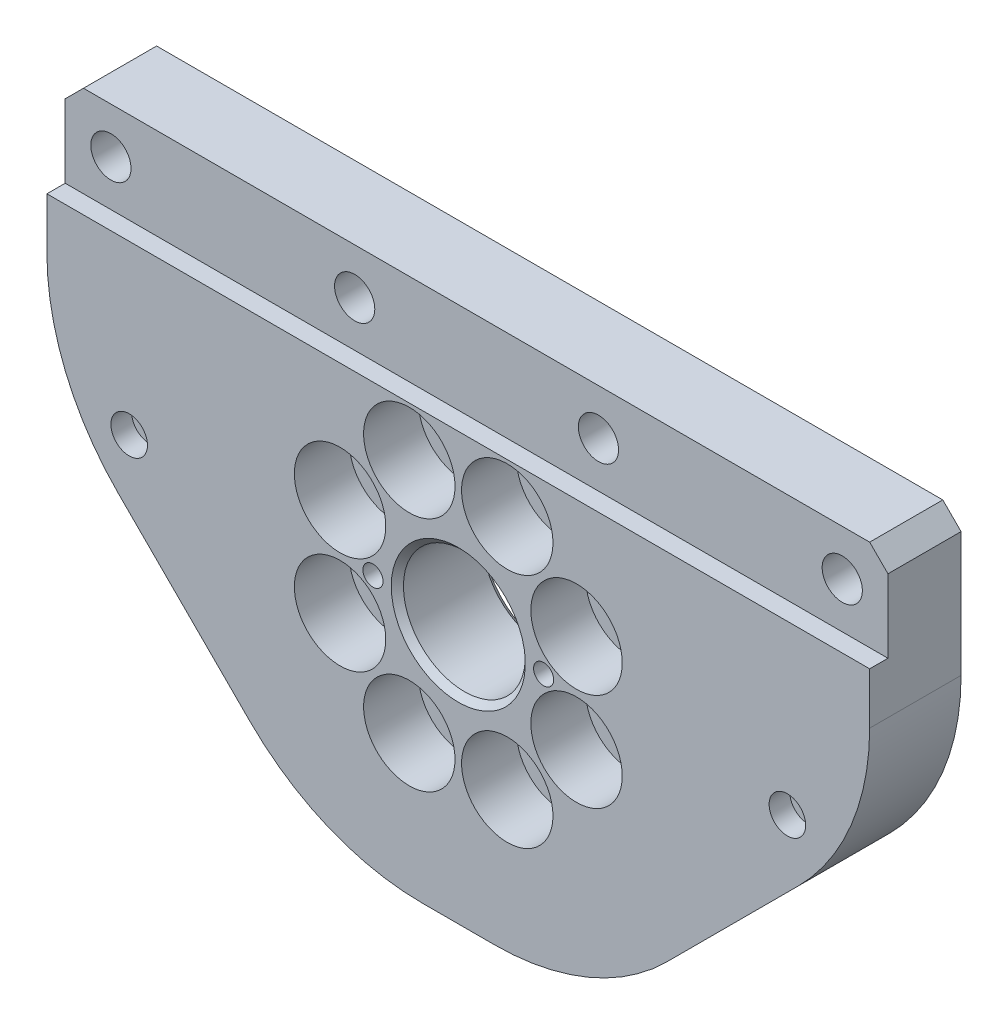
SolidWorks part; units mm, degrees
material "AL6061"
ref_plane "前视基准面" through (0, 0, 0) normal (0, 0, 1) x (1, 0, 0)
ref_plane "上视基准面" through (0, 0, 0) normal (0, 1, 0) x (1, 0, 0)
ref_plane "右视基准面" through (0, 0, 0) normal (1, 0, 0) x (0, 0, -1)
sketch "草图1" plane through (0, 0, 0) normal (0, 0, 1) x (1, 0, 0)
  line L0 (-77.8941, 0) -> (76.4, 0) construction
  line L1 (0, 37.9961) -> (0, -44.0164) construction
  line L2 (-55.7843, -9.2157) -> (-34.2157, -30.7843)
  line L3 (-67.5, 42.5) -> (67.5, 42.5)
  line L4 (-67.5, 42.5) -> (-67.5, 19.0685)
  line L5 (-5.9315, -42.5) -> (5.9315, -42.5)
  line L6 (67.5, 42.5) -> (67.5, 19.0685)
  line L7 (55.7843, -9.2157) -> (34.2157, -30.7843)
  arc A0 (-55.7843, -9.2157) -> (-67.5, 19.0685) centre (-27.5, 19.0685) cw
  arc A1 (-34.2157, -30.7843) -> (-5.9315, -42.5) centre (-5.9315, -2.5) ccw
  arc A2 (34.2157, -30.7843) -> (5.9315, -42.5) centre (5.9315, -2.5) cw
  arc A3 (55.7843, -9.2157) -> (67.5, 19.0685) centre (27.5, 19.0685) ccw
  circle A4 centre (0, 0) radius 10
  point P13 (-67.5, 2.5)
  point P16 (-22.5, -42.5)
  point P19 (22.5, -42.5)
  point P22 (67.5, 2.5)
  dimension "D5" = 40
  dimension "D6" = 42.5
  dimension "D7" = 20
  dimension "D1" = 135
  dimension "D2" = 85
  dimension "D3" = 45
  dimension "D4" = 45
extrude "凸台-拉伸1" add sketch "草图1" along normal mid plane 15
hole_wizard "打孔尺寸(%根据)内六角圆柱头螺钉的类型2" positions "草图2" profile "草图3" counterbore size "M8" standard "GB" end condition through all
sketch "草图2" plane through (0, 0, 7.5) normal (0, 0, 1) x (1, 0, 0)
  line L0 (0, 44.1868) -> (0, -47.6954) construction
  line L1 (0, 0) -> (-24.5604, 0) construction
  line L2 (0, 0) -> (-11.1113, 26.8251) construction
  circle A0 centre (0, 0) radius 21 construction
  point P0 (-8.0364, 19.4015)
  dimension "D1" = 42
  dimension "D2" = 22.5
sketch "草图3" plane through (-8.0364, 19.4015, 7.5) normal (1, 0, 0) x (0, -1, 0)
  line L0 (0, 0) -> (0, 15)
  line L1 (0, 15) -> (4.5, 15)
  line L3 (4.5, 15) -> (4.5, 9)
  line L4 (4.5, 9) -> (7.5, 9)
  line L5 (7.5, 9) -> (7.5, 0)
  line L7 (7.5, 0) -> (0, 0)
  line L11 (0, -6.35) -> (0, 107.95) construction
  dimension "通孔孔直径" = 9
  dimension "通孔孔深度" = 15
  dimension "柱形沉头孔直径" = 15
  dimension "柱形沉头孔深度" = 9
chamfer "倒角1" distance 1 angle 45 2 edges at (10, 0, -7.5) (10, 0, 7.5)
pattern_circular "阵列(圆周)1" count 8 over 360 about axis through (0, 0, 0) along (0, 0, 1) of "打孔尺寸(%根据)内六角圆柱头螺钉的类型2"
hole_wizard "打孔尺寸(%根据)内六角圆柱头螺钉的类型2" positions "草图4" profile "草图5" counterbore size "M3" standard "GB" end condition through all
sketch "草图4" plane through (0, 0, 7.5) normal (0, 0, 1) x (1, 0, 0)
  line L0 (0, 45.6613) -> (0, -51.3453) construction
  line L1 (0, 0) -> (80.3336, 0) construction
  point P0 (-54, 0)
  point P8 (54, 0)
  dimension "D1" = 108
sketch "草图5" plane through (-54, 0, 7.5) normal (1, 0, 0) x (0, -1, 0)
  line L0 (0, 0) -> (0, 15)
  line L1 (0, 15) -> (1.7, 15)
  line L3 (1.7, 15) -> (1.7, 3.4)
  line L4 (1.7, 3.4) -> (3, 3.4)
  line L5 (3, 3.4) -> (3, 0)
  line L7 (3, 0) -> (0, 0)
  line L11 (0, -6.35) -> (0, 107.95) construction
  dimension "通孔孔直径" = 3.4
  dimension "通孔孔深度" = 15
  dimension "柱形沉头孔直径" = 6
  dimension "柱形沉头孔深度" = 3.4
hole_wizard "Ø8.0 (8) 直径孔1" positions "草图6" profile "草图7" hole size "Ø8.0" standard "GB"
sketch "草图6" plane through (0, 0, -7.5) normal (0, 0, -1) x (-1, 0, 0)
  point P0 (-54, 0)
  point P3 (54, 0)
sketch "草图7" plane through (54, 0, -7.5) normal (1, 0, 0) x (0, 1, 0)
  line L0 (0, 0) -> (0, 10.4034)
  line L1 (0, 10.4034) -> (4, 8)
  line L2 (4, 8) -> (4, 0)
  line L5 (4, 0) -> (0, 0)
  line L10 (0, 10.4034) -> (-4, 8) construction
  line L11 (0, -6.35) -> (0, 107.95) construction
  dimension "孔直径" = 8
  dimension "孔深度" = 8
  dimension "导头角度" = 118
hole_wizard "M4 螺纹孔1" positions "草图8" profile "草图9" tap size "M4" standard "GB" end condition through all
sketch "草图8" plane through (0, 0, -7.5) normal (0, 0, -1) x (-1, 0, 0)
  line L0 (0, 0) -> (-34.4162, 0) construction
  line L1 (0, 22.5985) -> (0, -19.4015) construction
  point P0 (-14, 0)
  point P12 (14, 0)
  dimension "D1" = 28
sketch "草图9" plane through (14, 0, -7.5) normal (1, 0, 0) x (0, 1, 0)
  line L0 (0, 0) -> (0, 15)
  line L1 (0, 15) -> (1.65, 15)
  line L2 (1.65, 15) -> (1.65, 0)
  line L5 (1.65, 0) -> (0, 0)
  line L11 (0, -6.35) -> (0, 107.95) construction
  dimension "通孔螺纹孔钻头直径" = 3.3
  dimension "通孔螺纹孔钻头深度" = 15
cosmetic thread "孔螺蚊线1" parameters "D2"=4
cosmetic thread "孔螺蚊线2" parameters "D2"=4
sketch "草图10" plane through (0, 0, 7.5) normal (0, 0, 1) x (1, 0, 0)
  line L0 (67.5, 19.0685) -> (67.5, 42.5) construction
  line L1 (-67.5, 42.5) -> (67.5, 42.5)
  line L2 (-67.5, 42.5) -> (-67.5, 27.5)
  line L3 (-67.5, 27.5) -> (67.5, 27.5)
  line L4 (67.5, 42.5) -> (67.5, 27.5)
  dimension "D1" = 15
extrude "切除-拉伸1" cut sketch "草图10" against normal blind 3
hole_wizard "打孔尺寸(%根据)内六角圆柱头螺钉的类型3" positions "草图11" profile "草图12" counterbore size "M6" standard "GB" end condition through all
sketch "草图11" plane through (0, 0, -7.5) normal (0, 0, -1) x (-1, 0, 0)
  line L0 (0, 44.4035) -> (0, -4.632) construction
  line L1 (-67.5, 42.5) -> (67.5, 42.5) construction
  point P0 (-20, 35)
  point P2 (-60, 35)
  point P9 (60, 35)
  point P10 (20, 35)
  dimension "D1" = 40
  dimension "D2" = 120
  dimension "D3" = 7.5
sketch "草图12" plane through (20, 35, -7.5) normal (1, 0, 0) x (0, 1, 0)
  line L0 (0, 0) -> (0, 15)
  line L1 (0, 15) -> (3.3, 15)
  line L3 (3.3, 15) -> (3.3, 6.8)
  line L4 (3.3, 6.8) -> (5.5, 6.8)
  line L5 (5.5, 6.8) -> (5.5, 0)
  line L7 (5.5, 0) -> (0, 0)
  line L11 (0, -6.35) -> (0, 107.95) construction
  dimension "通孔孔直径" = 6.6
  dimension "通孔孔深度" = 15
  dimension "柱形沉头孔直径" = 11
  dimension "柱形沉头孔深度" = 6.8
chamfer "倒角2" distance 3 angle 45 2 edges at (-67.5, 42.5, -1.5) (67.5, 42.5, -1.5)
